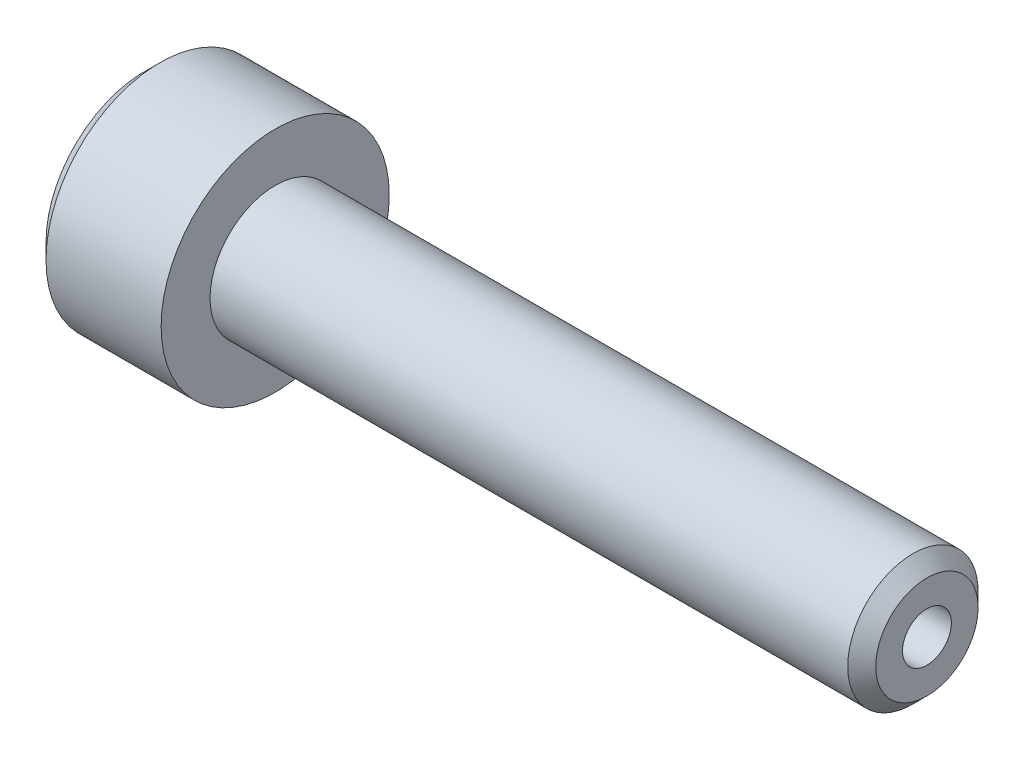
SolidWorks part; units mm, degrees
ref_plane "Front Plane" through (0, 0, 0) normal (0, 0, 1) x (1, 0, 0)
ref_plane "Top Plane" through (0, 0, 0) normal (0, 1, 0) x (1, 0, 0)
ref_plane "Right Plane" through (0, 0, 0) normal (1, 0, 0) x (0, 0, -1)
sketch "Sketch1" plane through (0, 0, 0) normal (0, 0, 1) x (1, 0, 0)
  line L0 (-4, 0) -> (-4, 3.0333)
  line L1 (-4, 3.0333) -> (-3.5333, 3.5)
  line L2 (-3.5333, 3.5) -> (0, 3.5)
  line L3 (0, 3.5) -> (0, 2)
  line L4 (0, 2) -> (19.57, 2)
  line L5 (19.57, 2) -> (20, 1.57)
  line L6 (20, 1.57) -> (20, 0)
  line L7 (20, 0) -> (-4, 0)
  line L8 (20, 0) -> (-4, 0) construction
revolve "Revolve1" add sketch "Sketch1" angle 360 about L8
cosmetic thread "Cosmetic Thread1" parameters "D1"=19.2552, "D2"=3.1399
sketch "Sketch2" plane through (0, 0, 0) normal (0, 0, 1) x (1, 0, 0)
  line L0 (-4, 0) -> (-4, 1.5)
  line L1 (-4, 1.5) -> (-2, 1.5)
  line L2 (-2, 1.5) -> (-1.727, 0.75)
  line L3 (-1.727, 0.75) -> (20, 0.75)
  line L4 (20, 0.75) -> (20, 0)
  line L5 (20, 0) -> (-4, 0)
  line L6 (20, 0) -> (-4, 0) construction
revolve "Cut-Revolve1" cut sketch "Sketch2" angle 360 about L6
ref_plane "Plane1" through (-4, 0, 0) normal (1, 0, 0) x (0, 0, -1)
sketch "Sketch3" plane through (-4, 0, 0) normal (1, 0, 0) x (0, 0, -1)
  line L0 (-1.5, 0.866) -> (-1.5, -0.866)
  line L1 (-1.5, -0.866) -> (0, -1.7321)
  line L2 (0, -1.7321) -> (1.5, -0.866)
  line L3 (1.5, -0.866) -> (1.5, 0.866)
  line L4 (1.5, 0.866) -> (0, 1.7321)
  line L5 (0, 1.7321) -> (-1.5, 0.866)
extrude "Cut-Extrude1" cut sketch "Sketch3" along normal blind 2
